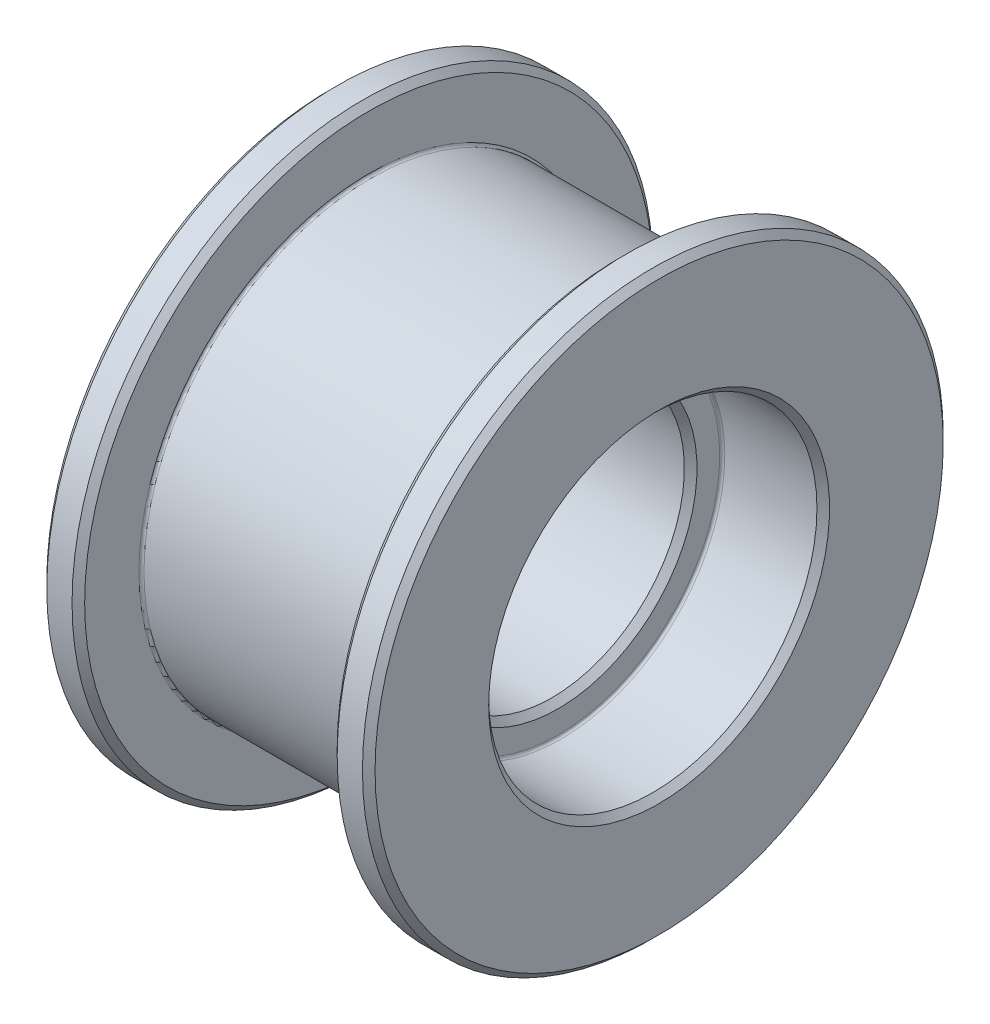
from build123d import *

# Parameters (mm, degrees)
CHAMFER_1_SIZE = 0.5
FILLET_1_R     = 0.2


with BuildPart() as part:
    # 草图1 → 旋转1 (revolve)
    with BuildSketch(Plane.XY, mode=Mode.PRIVATE) as revolve_1_sk:
        Polygon((-13, 13), (-13, 23), (-10, 23), (-10, 18), (10, 18), (10, 23), (13, 23), (13, 13), (5, 13), (5, 10.5), (-5, 10.5), (-5, 13), align=None)
    revolve(revolve_1_sk.sketch.rotate(Axis((0, 0, 0), (1, 0, 0)), 90), axis=Axis((0, 0, 0), (1, 0, 0)))

    # 倒角1
    chamfer_1_edges = [part.edges().sort_by_distance(p)[0] for p in [
        (13, 0, -13),
        (13, 0, -23),
        (10, 0, -23),
        (-10, 0, -23),
        (-13, 0, -23),
        (-13, 0, -13),
        (-5, 0, -10.5),
        (5, 0, -10.5),
    ]]
    chamfer(chamfer_1_edges, length=CHAMFER_1_SIZE)

    # 圆角1
    fillet_1_edges = [part.edges().sort_by_distance(p)[0] for p in [
        (10, 0, -18),
        (-10, 0, -18),
        (-5, 0, -13),
        (5, 0, -13),
    ]]
    fillet(fillet_1_edges, radius=FILLET_1_R)


solid = part.part
